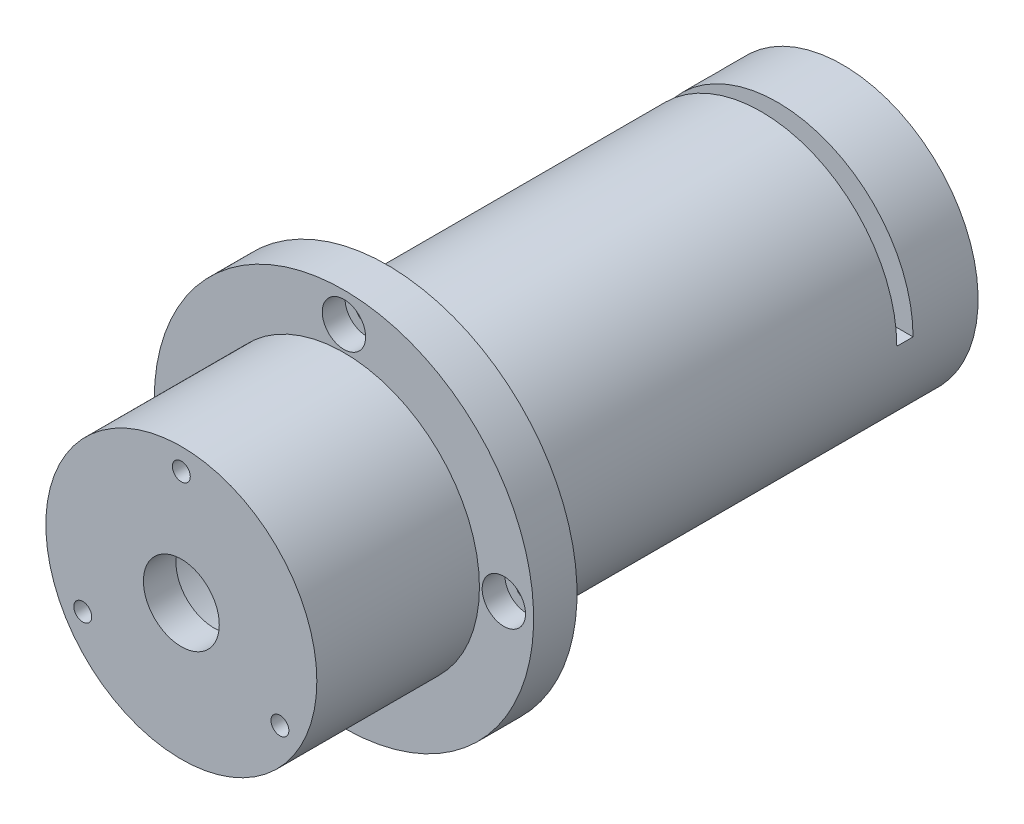
SolidWorks part; units mm, degrees
material "6061 合金"
ref_plane "前视基准面" through (0, 0, 0) normal (0, 0, 1) x (1, 0, 0)
ref_plane "上视基准面" through (0, 0, 0) normal (0, 1, 0) x (1, 0, 0)
ref_plane "右视基准面" through (0, 0, 0) normal (1, 0, 0) x (0, 0, -1)
sketch "草图2" plane through (0, 0, 0) normal (0, 0, 1) x (1, 0, 0)
  circle A0 centre (0, 0) radius 35
  dimension "D1" = 70
extrude "凸台-拉伸1" add sketch "草图2" along normal blind 122
sketch "草图3" plane through (0, 0, 122) normal (0, 0, 1) x (1, 0, 0)
  circle A0 centre (0, 0) radius 7
  dimension "D1" = 14
extrude "切除-拉伸1" cut sketch "草图3" against normal through all
sketch "草图4" plane through (0, 0, 0) normal (0, 0, -1) x (-1, 0, 0)
  circle A0 centre (0, 0) radius 17.5
  dimension "D1" = 35
extrude "切除-拉伸2" cut sketch "草图4" against normal blind 116
sketch "草图5" plane through (0, 0, 122) normal (0, 0, 1) x (1, 0, 0)
  circle A0 centre (0, 0) radius 25
  dimension "D1" = 50
extrude "切除-拉伸3" cut sketch "草图5" against normal blind 30 flip side to cut
sketch "草图6" plane through (0, 0, 0) normal (0, 0, -1) x (-1, 0, 0)
  circle A0 centre (0, 0) radius 25
  dimension "D1" = 50
extrude "切除-拉伸4" cut sketch "草图6" against normal blind 84 flip side to cut
sketch "草图7" plane through (0, 0, 92) normal (0, 0, 1) x (1, 0, 0)
  line L0 (-45.1301, 0) -> (49.4147, 0) construction
  line L1 (0, 41.6419) -> (0, -43.7282) construction
  circle A0 centre (0, 0) radius 29.5 construction
  circle A1 centre (0, 29.5) radius 2.1
  circle A2 centre (29.5, 0) radius 2.1
  circle A3 centre (0, -29.5) radius 2.1
  circle A4 centre (-29.5, 0) radius 2.1
  dimension "D1" = 59
  dimension "D2" = 4.2
  dimension "D3" = 4.2
  dimension "D4" = 4.2
  dimension "D5" = 4.2
extrude "切除-拉伸5" cut sketch "草图7" against normal through all
sketch "草图8" plane through (0, 0, 92) normal (0, 0, 1) x (1, 0, 0)
  circle A0 centre (0, 29.5) radius 4
  circle A1 centre (-29.5, 0) radius 4
  circle A2 centre (29.5, 0) radius 4
  circle A3 centre (0, -29.5) radius 4
  dimension "D1" = 8
  dimension "D2" = 8
  dimension "D3" = 8
  dimension "D4" = 8
extrude "切除-拉伸6" cut sketch "草图8" against normal blind 4.2
sketch "草图9" plane through (0, 0, 122) normal (0, 0, 1) x (1, 0, 0)
  line L0 (0, 38.488) -> (0, -41.3232) construction
  line L1 (0, 0) -> (35.6315, -20.5719) construction
  line L2 (0, 0) -> (-35.2534, -20.3536) construction
  circle A0 centre (0, 0) radius 21 construction
  dimension "D1" = 42
  dimension "D2" = 120
  dimension "D3" = 120
hole_wizard "M4 螺纹孔1" positions "3D草图1" profile "草图10" tap size "M4" standard "GB"
sketch3d "3D草图1"
  line L0 (0, 0, 122) -> (35.6315, -20.5719, 122) construction
  line L1 (0, 0, 122) -> (-35.2534, -20.3536, 122) construction
  line L2 (0, 38.488, 122) -> (0, -41.3232, 122) construction
  circle A0 centre (0, 0, 122) radius 21 construction
  point P0 (17.8158, -10.2859, 122)
  point P4 (18.1865, -10.5, 122)
  point P8 (0, 0, 143)
  point P9 (-18.1865, -10.5, 122)
  point P13 (0, 21, 122)
sketch "草图10" plane through (18.1865, -10.5, 122) normal (1, 0, 0) x (0, -1, 0)
  line L0 (0, 0) -> (0, 11.4914)
  line L1 (0, 11.4914) -> (1.65, 10.5)
  line L2 (1.65, 10.5) -> (1.65, 0)
  line L5 (1.65, 0) -> (0, 0)
  line L10 (0, 11.4914) -> (-1.65, 10.5) construction
  line L11 (0, -6.35) -> (0, 107.95) construction
  dimension "螺纹孔钻头直径" = 3.3
  dimension "螺纹孔钻头深度" = 10.5
  dimension "导头角度" = 118
cosmetic thread "孔螺蚊线1" parameters "D1"=7, "D2"=4
cosmetic thread "孔螺蚊线2" parameters "D1"=7, "D2"=4
cosmetic thread "孔螺蚊线3" parameters "D1"=7, "D2"=4
cosmetic thread "孔螺蚊线4" parameters "D1"=7, "D2"=4
sketch "草图19" plane through (0, 0, 0) normal (0, 0, -1) x (-1, 0, 0)
  line L0 (13.7548, 0) -> (45.9003, 0) construction
  line L1 (13.7548, 3) -> (26.6861, 3)
  line L2 (13.7548, 3) -> (13.7548, 0)
  line L3 (26.6861, 3) -> (26.6861, 0)
  line L4 (13.7548, 0) -> (26.6861, 0)
  line L5 (-43.6301, 3) -> (45.9003, 3) construction
  line L6 (-43.6301, 0) -> (45.9003, 0) construction
  dimension "D1" = 3
extrude "切除-拉伸7" cut sketch "草图19" against normal blind 15
ref_plane "基准面1" through (-25, 0, 0) normal (1, 0, 0) x (0, 0, -1)
sketch "草图20" plane through (-25, 0, 0) normal (1, 0, 0) x (0, 0, -1)
  line L0 (-15, 0) -> (-15, 28.4277)
  line L1 (-15, 28.4277) -> (-12, 28.4277)
  line L2 (-12, 28.4277) -> (-12, 0)
  line L3 (-12, 0) -> (-15, 0)
  dimension "D1" = 3
extrude "切除-拉伸8" cut sketch "草图20" along normal through all
ref_plane "基准面2" through (0, 25, 0) normal (0, 1, 0) x (-1, 0, 0)
sketch "草图21" plane through (0, 25, 0) normal (0, 1, 0) x (-1, 0, 0)
  line L0 (0, -33.7795) -> (0, 79.3603) construction
  line L2 (21, -33.7795) -> (21, 79.3603) construction
  line L3 (-25, 6) -> (25, 6)
  line L4 (-25, 6) -> (25, 6) construction
  circle A0 centre (21, 6) radius 4
  dimension "D3" = 8
  dimension "D1" = 6
  dimension "D2" = 21
extrude "切除-拉伸9" cut sketch "草图21" against normal blind 18
sketch "草图22" plane through (0, 25, 0) normal (0, 1, 0) x (-1, 0, 0)
  circle A0 centre (21, 6) radius 2.25
  dimension "D1" = 4.5
extrude "切除-拉伸10" cut sketch "草图22" against normal up to surface (22 mm away) up to face at (-21.0301, 3, 6)
sketch "草图24" plane through (0, 0, 0) normal (0, 1, 0) x (1, 0, 0)
  line L0 (-28.9818, -6) -> (-13.2888, -6) construction
  line L1 (-21, 1.9827) -> (-21, -13.9022) construction
hole_wizard "M4 螺纹孔3" positions "3D草图4" profile "草图26" tap size "M4" standard "GB" end condition through all
sketch3d "3D草图4"
  line L0 (-21, 0, -1.9827) -> (-21, 0, 13.9022) construction
  line L1 (-28.9818, 0, 6) -> (-13.2888, 0, 6) construction
  point P0 (-21, 0, 6)
  dimension "D1" = 0
sketch "草图26" plane through (-21, 0, 6) normal (1, 0, 0) x (0, 0, 1)
  line L0 (0, 0) -> (0, 35)
  line L1 (0, 35) -> (1.65, 35)
  line L2 (1.65, 35) -> (1.65, 0)
  line L5 (1.65, 0) -> (0, 0)
  line L11 (0, -6.35) -> (0, 107.95) construction
  dimension "通孔螺纹孔钻头直径" = 3.3
  dimension "通孔螺纹孔钻头深度" = 35
cosmetic thread "孔螺蚊线6" parameters "D2"=4
